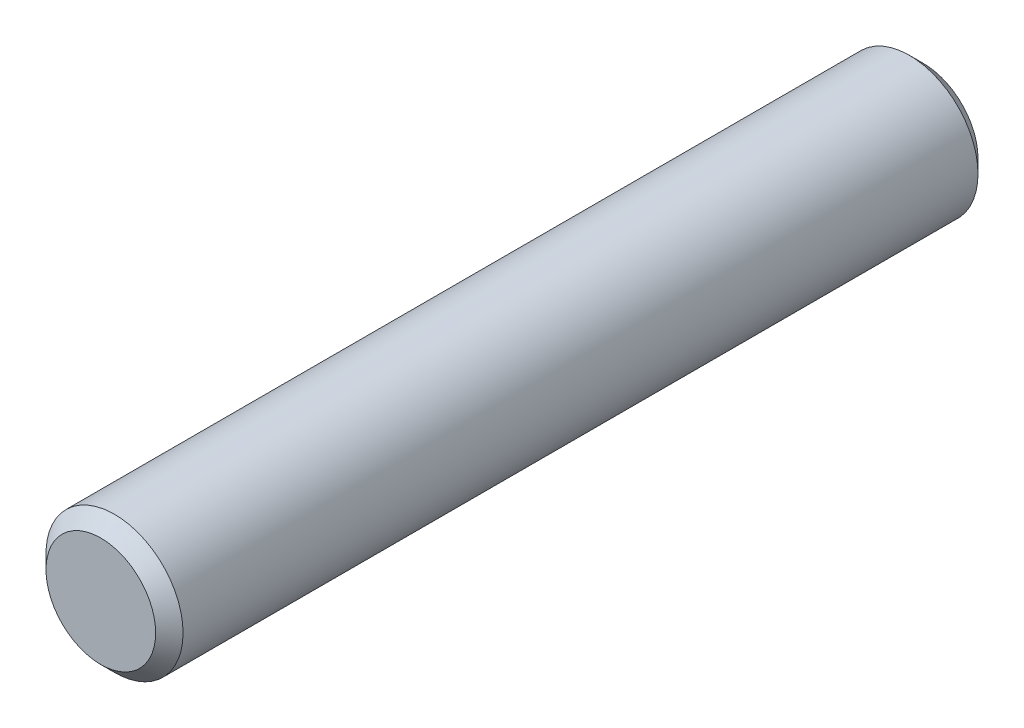
SolidWorks part; units mm, degrees
ref_plane "Front Plane" through (0, 0, 0) normal (0, 0, 1) x (1, 0, 0)
ref_plane "Top Plane" through (0, 0, 0) normal (0, 1, 0) x (1, 0, 0)
ref_plane "Right Plane" through (0, 0, 0) normal (1, 0, 0) x (0, 0, -1)
sketch "Sketch1" plane through (0, 0, 0) normal (0, 0, 1) x (1, 0, 0)
  circle A0 centre (0, 0) radius 2.5
  dimension "D1" = 5
extrude "Boss-Extrude1" add sketch "Sketch1" along normal mid plane 30
chamfer "Chamfer1" distance 0.5 angle 45 2 edges at (2.5, 0, 15) (2.5, 0, -15)
